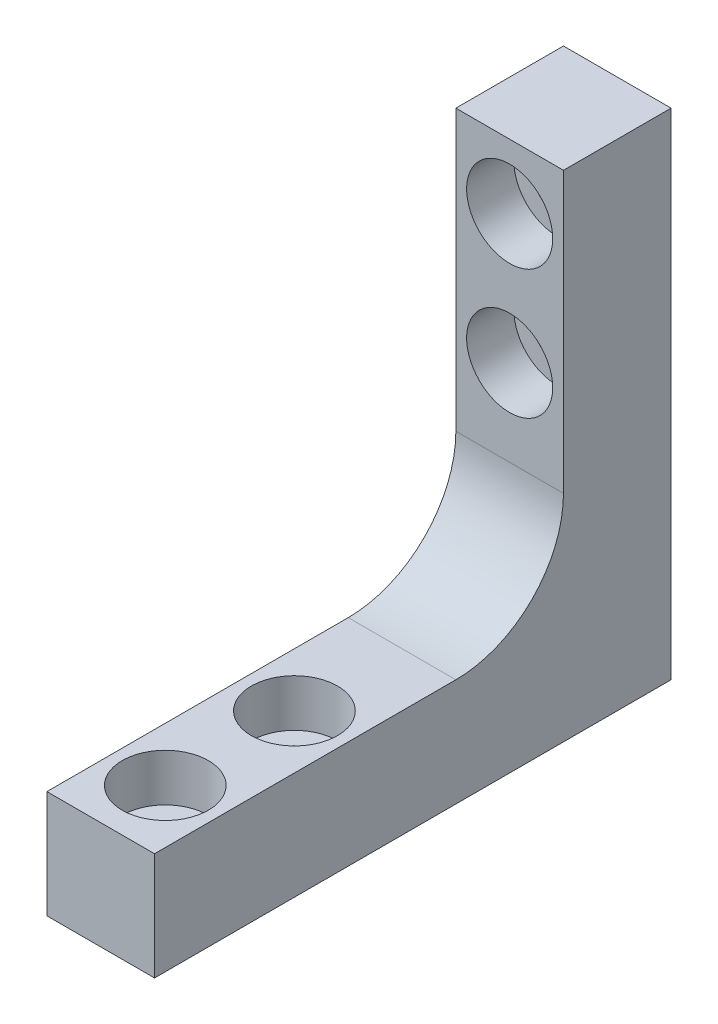
SolidWorks part; units mm, degrees
ref_plane "Front Plane" through (0, 0, 0) normal (0, 0, 1) x (1, 0, 0)
ref_plane "Top Plane" through (0, 0, 0) normal (0, 1, 0) x (1, 0, 0)
ref_plane "Right Plane" through (0, 0, 0) normal (1, 0, 0) x (0, 0, -1)
sketch "Sketch1" plane through (0, 0, 0) normal (1, 0, 0) x (0, 0, -1)
  line L1 (-24, 23) -> (24, 23)
  line L2 (-24, 23) -> (-24, -23)
  line L3 (-24, -23) -> (24, -23)
  line L4 (24, 23) -> (24, -23)
  line L5 (-24, 23) -> (24, -23) construction
  line L6 (-24, -23) -> (24, 23) construction
  point P0 (0, 0)
  dimension "D1" = 48
  dimension "D2" = 46
extrude "Boss-Extrude1" add sketch "Sketch1" along normal mid plane 10
sketch "Sketch2" plane through (5, 0, 0) normal (1, 0, 0) x (0, 0, -1)
  line L0 (-24, -23) -> (24, -23) construction
  line L1 (-24, 23) -> (14, 23)
  line L2 (-24, 23) -> (-24, -13)
  line L3 (-24, -13) -> (14, -13)
  line L4 (14, 23) -> (14, -13)
  line L5 (24, -23) -> (24, 23) construction
  dimension "D1" = 10
  dimension "D2" = 10
extrude "Cut-Extrude1" cut sketch "Sketch2" against normal through all
fillet "Fillet1" radius 10 1 edges at (0, -13, -14)
hole_wizard "CBORE for M4 Hex Socket Head Cap Screw1" positions "Sketch3" profile "Sketch4" counterbore size "M4" standard "ISO" end condition through all
sketch "Sketch3" plane through (0, -13, 0) normal (0, 1, 0) x (1, 0, 0)
  line L0 (-5, -24) -> (5, -24) construction
  line L1 (0, 0) -> (0, 10.191) construction
  point P0 (0, -18)
  point P2 (0, -6)
  dimension "D1" = 6
  dimension "D2" = 12
sketch "Sketch4" plane through (0, -13, 18) normal (1, 0, 0) x (0, 0, 1)
  line L0 (0, 0) -> (0, 10)
  line L1 (0, 10) -> (2.25, 10)
  line L3 (2.25, 10) -> (2.25, 4.4)
  line L4 (2.25, 4.4) -> (4, 4.4)
  line L5 (4, 4.4) -> (4, 0)
  line L7 (4, 0) -> (0, 0)
  line L11 (0, -6.35) -> (0, 107.95) construction
  dimension "通孔孔直径" = 4.5
  dimension "通孔孔深度" = 10
  dimension "柱形沉头孔直径" = 8
  dimension "柱形沉头孔深度" = 4.4
hole_wizard "CBORE for M4 Hex Socket Head Cap Screw2" positions "Sketch5" profile "Sketch6" counterbore size "M4" standard "ISO" end condition through all
sketch "Sketch5" plane through (0, 0, -14) normal (0, 0, 1) x (1, 0, 0)
  line L0 (-5, 23) -> (5, 23) construction
  point P0 (0, 17)
  point P2 (0, 5)
  dimension "D1" = 6
  dimension "D2" = 12
sketch "Sketch6" plane through (0, 17, -14) normal (1, 0, 0) x (0, -1, 0)
  line L0 (0, 0) -> (0, 10)
  line L1 (0, 10) -> (2.25, 10)
  line L3 (2.25, 10) -> (2.25, 4.4)
  line L4 (2.25, 4.4) -> (4, 4.4)
  line L5 (4, 4.4) -> (4, 0)
  line L7 (4, 0) -> (0, 0)
  line L11 (0, -6.35) -> (0, 107.95) construction
  dimension "通孔孔直径" = 4.5
  dimension "通孔孔深度" = 10
  dimension "柱形沉头孔直径" = 8
  dimension "柱形沉头孔深度" = 4.4
